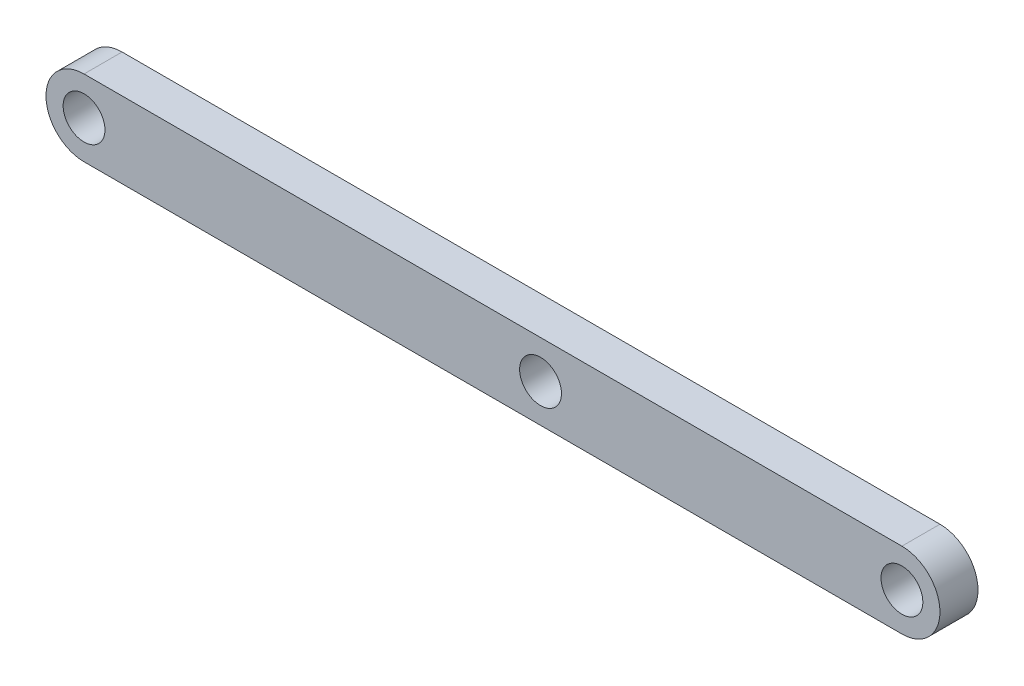
from build123d import *

# Parameters (mm, degrees)
SKETCH1_R           = 0.55
THIGH1_LENGTH_DEPTH = 0.5


with BuildPart() as part:
    # Sketch1 → Thigh1 length (new, symmetric)
    with BuildSketch(Plane.XY):
        with BuildLine():
            Line((-10.75, 1), (10.75, 1))
            ThreePointArc((10.75, 1), (11.75, 0), (10.75, -1))
            Line((10.75, -1), (-10.75, -1))
            ThreePointArc((-10.75, -1), (-11.75, 0), (-10.75, 1))
        make_face()
        with Locations((-10.75, 0)):
            Circle(SKETCH1_R, mode=Mode.SUBTRACT)
        with Locations((10.75, 0)):
            Circle(SKETCH1_R, mode=Mode.SUBTRACT)
        with Locations((1.25, 0)):
            Circle(SKETCH1_R, mode=Mode.SUBTRACT)
    extrude(amount=THIGH1_LENGTH_DEPTH, both=True)


solid = part.part
